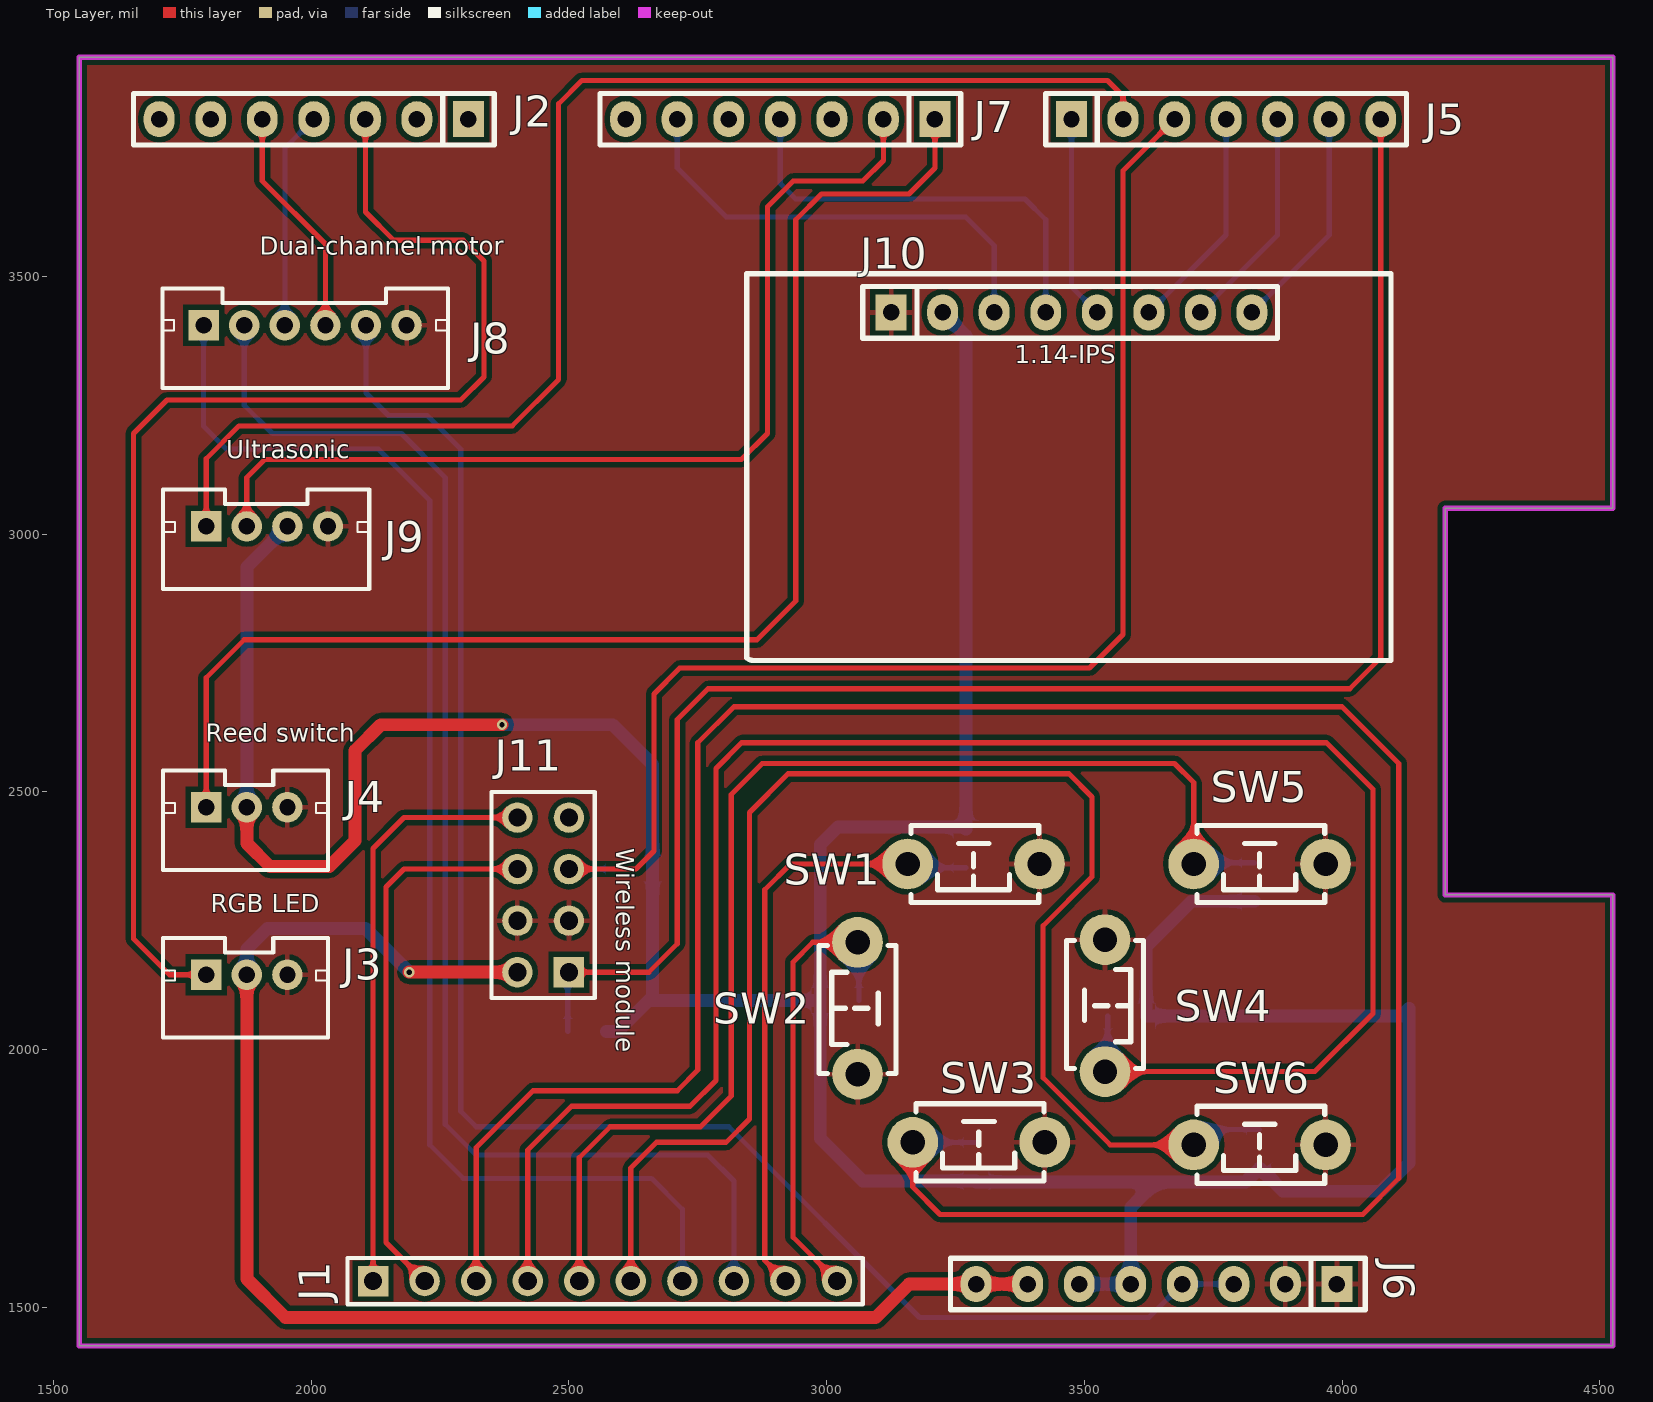
[diagram p0: Top Layer view]
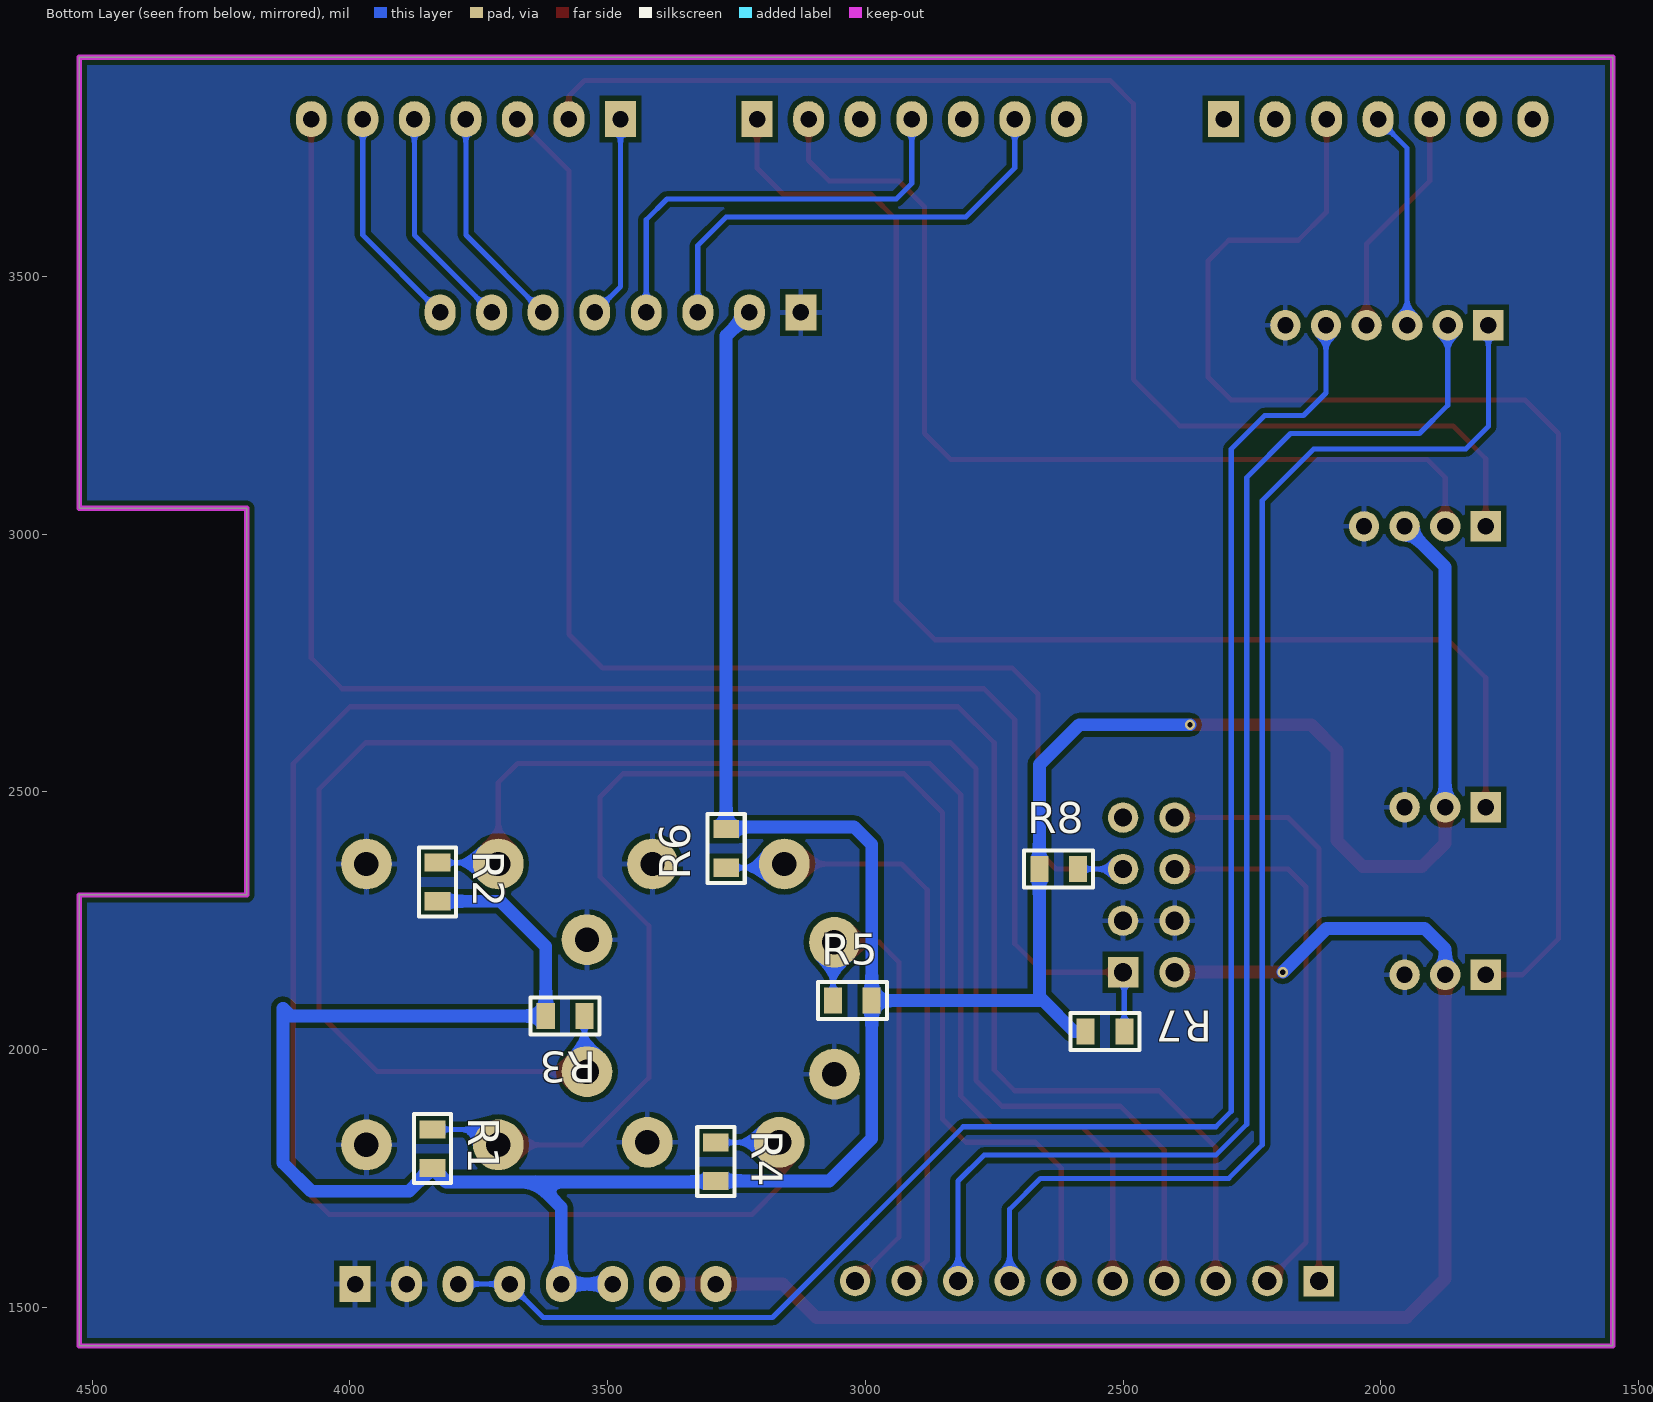
[diagram p1: Bottom Layer view, seen from below]
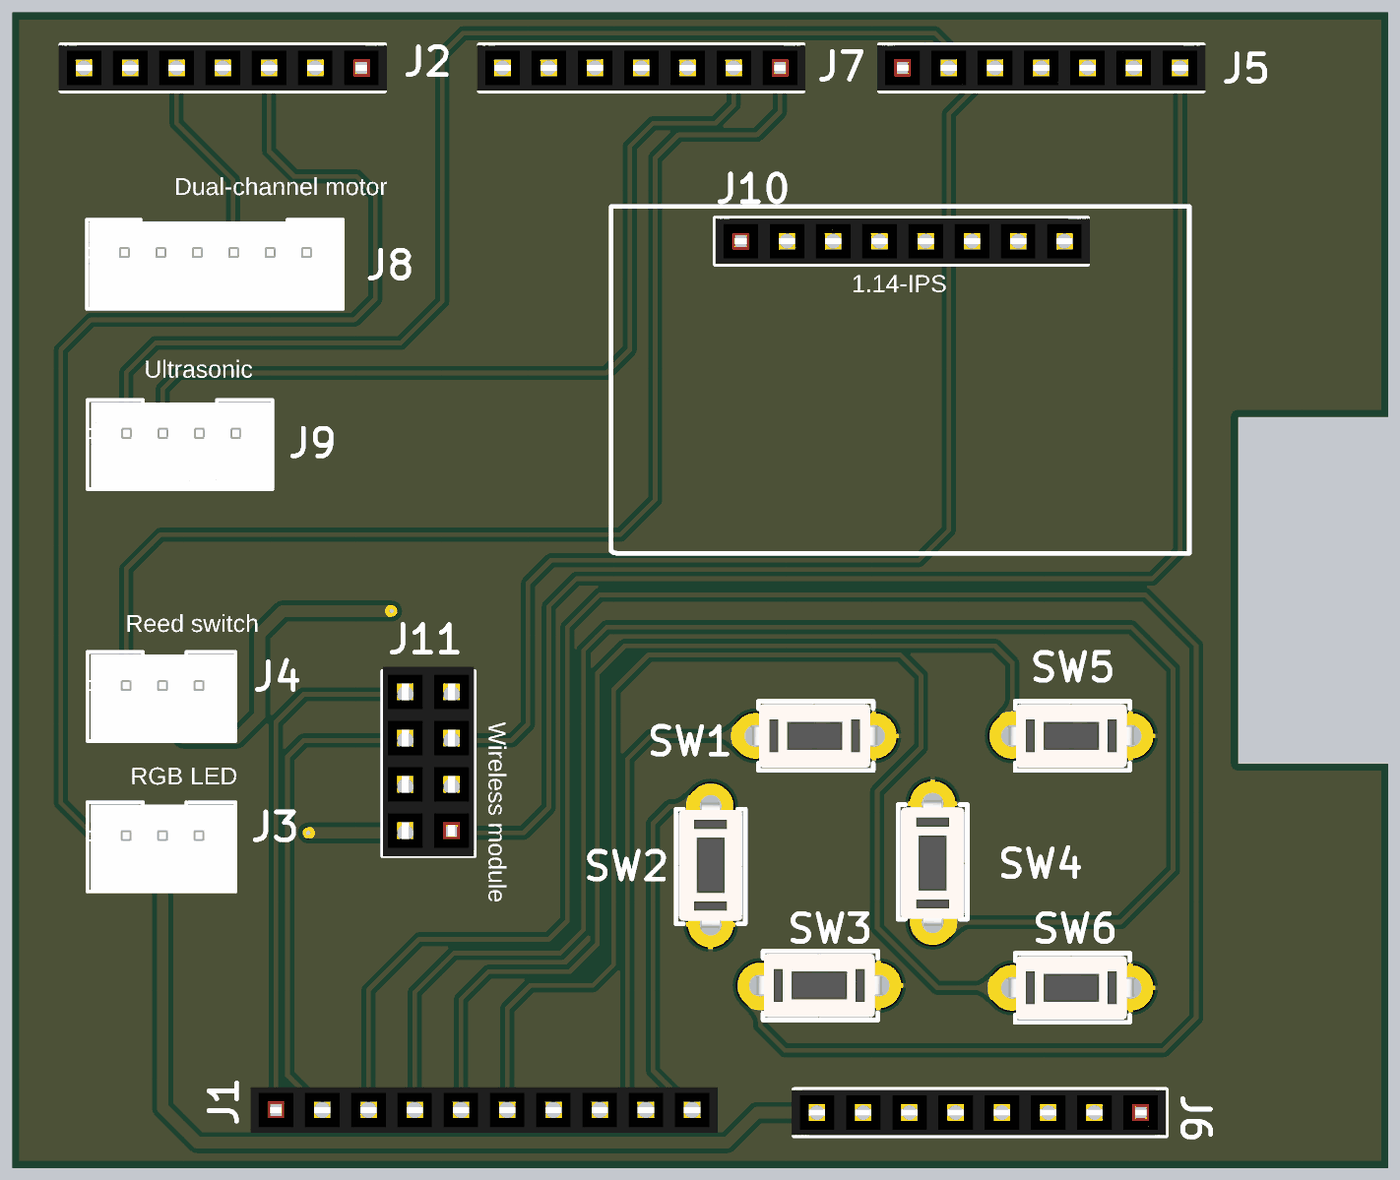
[diagram p2: 3D render of the assembled board from above, using the file's embedded part models]
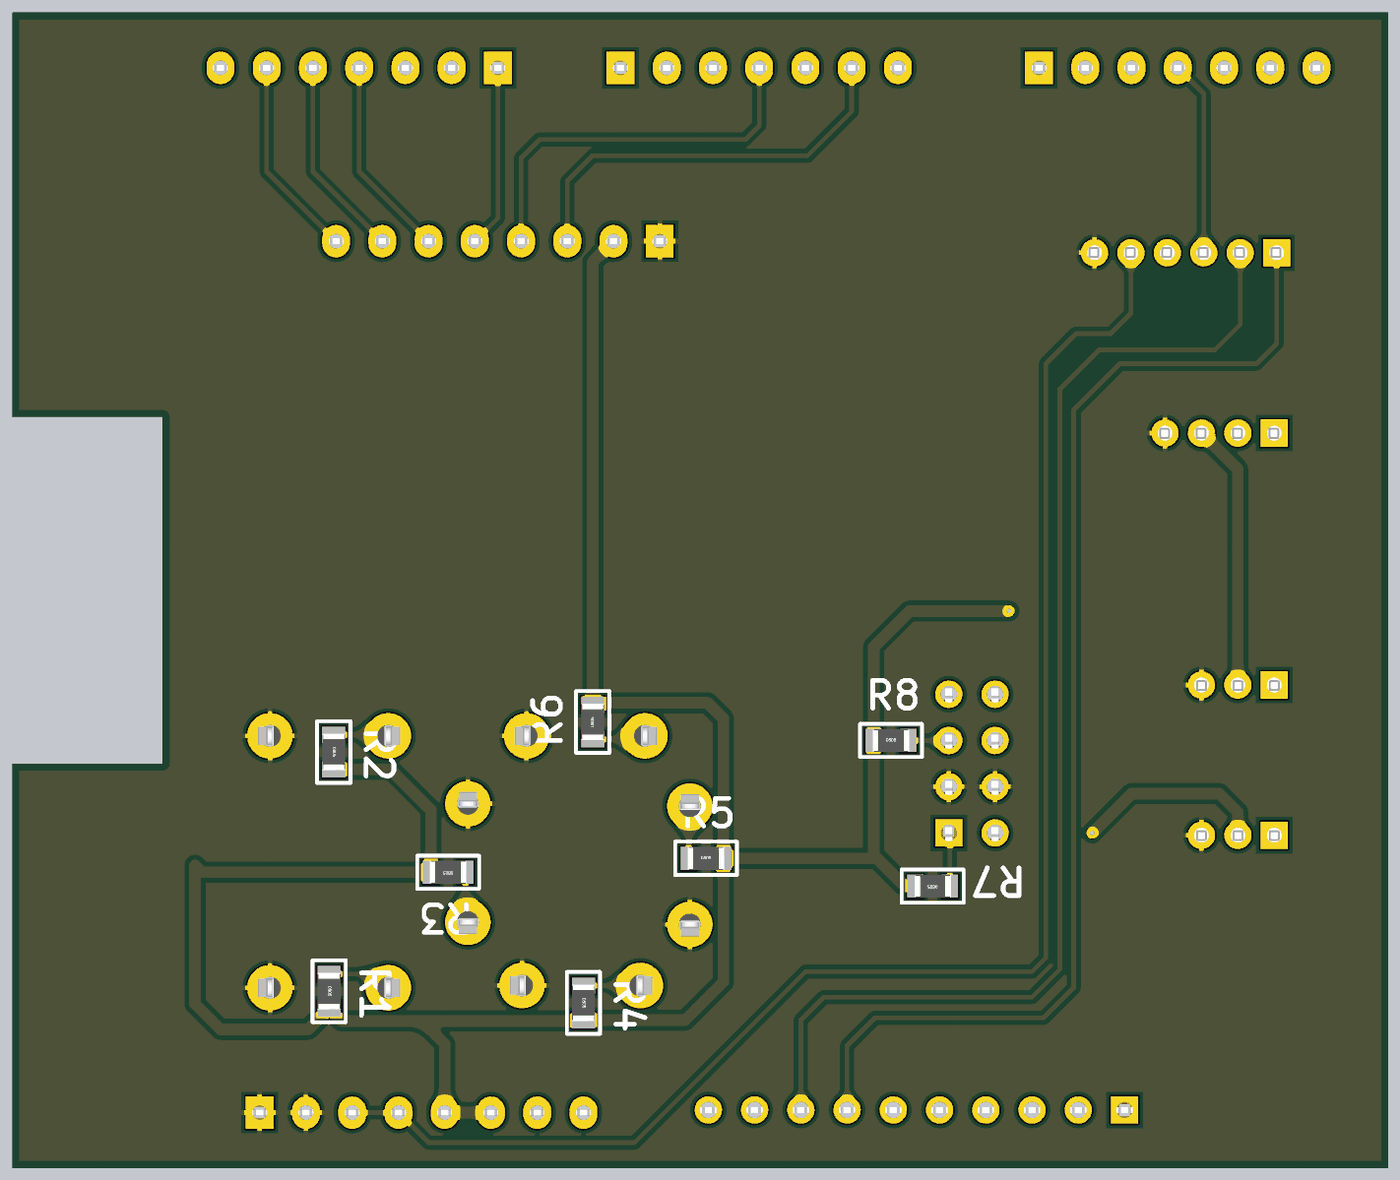
[diagram p3: 3D render of the assembled board from below, using the file's embedded part models]
# Altium PCB MISC80620.PcbDoc
Units mil, origin at the board's own origin, x right, y up, seen from the top; angles counter-clockwise.
Board outline 2975 x 2500 mil, 2 copper layers (Top Layer, Bottom Layer); 25 components, 35 nets, 99 pads, 2 vias.

## Layer stack, top to bottom (the 12.6 mil dielectric is the usual default, probably not edited)
Top Solder: solder mask 0.4, Solder Resist, Dk 3.5
Top Layer: signal copper 1.4
Dielectric 1: dielectric 12.6, FR-4, Dk 4.8
Bottom Layer: signal copper 1.4
Bottom Solder: solder mask 0.4, Solder Resist, Dk 3.5

## Board outline
1550,1425 1550,3925 4525,3925 4525,3050 4200,3050 4200,2300 4525,2300 4525,1425

## Design rules (kind name [scope] priority, off if disabled: settings)
Clearance [All] p1: gap=10
MinimumSolderMaskSliver [All] p1: minsoldermaskwidth=0
PolygonConnect [All] p1: connectstyle=Relief reliefconductorwidth=10 reliefentries=4 polygonreliefangle="90 Angle" airgapwidth=10
RoutingVias [All] p1: holewidth=28 width=50 viastyle="Through Hole" minholewidth=28 minwidth=50 maxholewidth=28 maxwidth=50
SilkToSilkClearance [All] p1: silktosilkclearance=0
SilkToSolderMaskClearance [IsPad] p1: minsilkscreentomaskgap=0 clearancetoexposedcopper=TRUE
SolderMaskExpansion [All] p1: expansion=4
Width [All] p1: maxlimit=30 minlimit=10 preferedwidth=10
27 further rules are at their usual default settings.

## Components (designator, comment, footprint, x,y, rotation, side; value= is the part's Value field where it differs from the comment)
J1 "Female HDR1X10" Fe-HDR1X10/2.54-S 2120,1550.78 r90 top
J2 "Female HDR1X7" Fe-HDR1X7/2.54-S 2305,3805 r270 top
J3 "PH2.0-3P" PH2.0-3P 1796.26,2145 r0 top
J4 "PH2.0-3P" PH2.0-3P 1796.26,2470 r0 top
J5 "Female HDR1X7" Fe-HDR1X7/2.54-S 3475,3805 r90 top
J6 "Female HDR1X8" Fe-HDR1X8/2.54-S 3990,1545 r270 top
J7 "Female HDR1X7" Fe-HDR1X7/2.54-S 3210,3805 r270 top
J8 "PH2.0-6P" PH2.0-6P 1791.26,3405 r0 top
J9 "PH2.0-4P" PH2.0-4P 1796.26,3015 r0 top
J10 "CON8" Fe-HDR1X8/2.54-S 3125,3430 r90 top
J11 "Female HDR2X4" Fe-HDR2X4/2.54-S 2500,2150 r90 top
R1 "4.7K" "R 0805_L" 3840,1807.6 r270 bottom
R2 "4.7K" "R 0805_L" 3830,2325 r270 bottom
R3 "4.7K" "R 0805_L" 3582.6,2065 r0 bottom
R4 "4.7K" "R 0805_L" 3290,1782.4 r270 bottom
R5 "4.7K" "R 0805_L" 3025,2095 r180 bottom
R6 "4.7K" "R 0805_L" 3270,2390 r90 bottom
R7 "10K" "R 0805_L" 2535,2035 r0 bottom
R8 "10K" "R 0805_L" 2625,2350 r180 bottom
SW1 "3x6x5" "TSW DIP-3*6*4.3" 3285,2360 r180 top
SW2 "3x6x5" "TSW DIP-3*6*4.3" 3060,2080 r90 top
SW3 "3x6x5" "TSW DIP-3*6*4.3" 3295,1820 r180 top
SW4 "3x6x5" "TSW DIP-3*6*4.3" 3540,2085 r270 top
SW5 "3x6x5" "TSW DIP-3*6*4.3" 3840,2360 r180 top
SW6 "3x6x5" "TSW DIP-3*6*4.3" 3840,1815 r180 top

## Footprints (in the part's own frame and the unit in brackets; to place one, negate y for a bottom-side part, rotate by r counter-clockwise, add the part's x,y. Pads: shape width x height; smd on the part's side, far side on the other; paste and mask are expansions set on the pad)
Fe-HDR1X7/2.54-S [mil]
  rect 70x60 hole 32: 1(0,0)
  oval 70x60 hole 32: 2(0,-100) 3(0,-200) 4(0,-300) 5(0,-400) 6(0,-500) 7(0,-600)
  silkscreen extent -50,-650 50,50, body extent -49,-655 49,55, height 126
Fe-HDR1X8/2.54-S [mil]
  rect 70x60 hole 32: 1(0,0)
  oval 70x60 hole 32: 2(0,-100) 3(0,-200) 4(0,-300) 5(0,-400) 6(0,-500) 7(0,-600) 8(0,-700)
  silkscreen extent -50,-750 50,55, body extent -49,-755 49,55, height 126
Fe-HDR1X10/2.54-S [mm]
  rect 1.5x1.5 hole 0.9: 1(0,0)
  round 1.5 hole 0.9: 2(0,-2.54) 3(0,-5.08) 4(0,-7.62) 5(0,-10.16) 6(0,-12.7) 7(0,-15.24) 8(0,-17.78) 9(0,-20.32) 10(0,-22.86)
  silkscreen extent -1.14,-24.13 1.14,1.27, body extent -1.25,-24.26 1.25,1.4, height 3.2
Fe-HDR2X4/2.54-S [mm] "Connector; Header; 4x2 Position"
  rect 1.5x1.5 hole 0.9: 1(0,0)
  round 1.5 hole 0.9: 2(0,2.54) 3(2.54,0) 4(2.54,2.54) 5(5.08,0) 6(5.08,2.54) 7(7.62,0) 8(7.62,2.54)
  silkscreen extent -1.27,-1.27 8.89,3.81, body extent -1.27,-1.23 9.14,3.77, height 8.5
PH2.0-3P [mm]
  rect 1.5x1.5 hole 0.8: 1(0,0)
  round 1.5 hole 0.8: 2(2,0) 3(4,0)
  silkscreen extent -2.13,-3.08 6,1.82, body extent -1.95,-3.02 5.95,1.68, height 6.01
PH2.0-4P [mm]
  rect 1.5x1.5 hole 0.8: 1(0,0)
  round 1.5 hole 0.8: 2(2,0) 3(4,0) 4(6,0)
  silkscreen extent -2.13,-3.08 8.03,1.82, body extent -1.93,-3.01 7.97,1.69, height 6.01
PH2.0-6P [mm]
  rect 1.5x1.5 hole 0.8: 1(0,0)
  round 1.5 hole 0.8: 2(2,0) 3(4,0) 4(6,0) 5(8,0) 6(10,0)
  silkscreen extent -2.03,-3.08 12.03,1.82, body extent -1.91,-2.98 11.99,1.71, height 6.01
"R 0805_L" [mil] "1/8W贴片电阻"
  rect 35x50 smd: 1(-37.4,0) 2(37.4,0)
  silkscreen extent -67,-36 67,36, body extent -39,-25 39,25, height 20
"TSW DIP-3*6*4.3" [mm] "3*6*4.3mm"
  round 2.5 hole 1.2: 1(3.25,0) 2(-3.25,0)
  silkscreen extent -3.21,-1.9 3.09,1.9, body extent -3.91,-1.75 3.91,1.75, height 4.31

## Part data
J10: library part "Female HDR1X8"
R1 R2 R3 R4 R5 R6 R7 R8: library part R, "SMD resistor"
SW1 SW2 SW3 SW4 SW5 SW6: library part "TSW 3x6", "3x6 tact switch"

## Via types
v1: diameter 20, hole 10, Top Layer to Bottom Layer, 2 vias

## Nets (pads, with @x,y where several pads share a name; then routed paths per layer and width w, separated by ;. In a path a pad name is that pad's centre, name@x,y a point inside that pad or via, vN(x,y) a via of type N, cw(c..) or ccw(c..) an arc to the next point about the centre after c; other vN are vias at no path point)
3V3: J4.2 J6.5 J6.6 J9.3 J10.2 R1.2 R2.2 R3.2 R4.2 R5.2 R6.2 R7.2 R8.1 | length 7240
  Top Layer w25: J4.2 1875,2400 1920,2355 2035,2355 2085,2405 2085,2580 2135,2630 v1(2370,2630)
  Bottom Layer w25: J4.2 1875,2936.26 J9.3 ; v1(2370,2630) 2585,2630 2662.4,2552.6 R8.1 2662.4,2102.4 2655,2095 ; R7.2 2595,2035 2655,2095 ; J10.2 3270,3385 R6.2 3265.68,2431.71 3021.71,2431.71 2987.6,2397.6 R5.2 ; J6.6 J6.5 3590,1693.29 3640,1743.29 ; R2.2 3707.6,2287.6 3620,2200 R3.2 4115,2065 4130,2080 4130,1780 4075,1725 3885.2,1725 R1.2 3813.09,1743.29 3640,1743.29 ; 2655,2095 R5.2 ; R5.2 2987.6,1827.4 3070,1745 R4.2 3290,1743.29 3640,1743.29
5V: J3.2 J6.7 J6.8 J11.2 | length 2789.8
  Top Layer w25: J3.2 1875,1555 1950,1480 3095,1480 3160,1545 J6.8 J6.7 ; v1(2190,2150) J11.2
  Bottom Layer w25: J3.2 1875,2195 1915,2235 2105,2235 v1(2190,2150)
A0: J1.7 J8.1 | length 2625.5
  Bottom Layer w10: J8.1 1791.26,3208.74 1835,3165 2130,3165 2230,3065 2230,1815 2295,1750 2660,1750 2720,1690 J1.7
A1: J1.8 J8.2 | length 2657.8
  Bottom Layer w10: J8.2 1870,3250 1925,3195 2175,3195 2260,3110 2260,1855 2320,1795 2770,1795 2820,1745 J1.8
A4: J1.9 R6.1 SW1.1 | length 1189.6
  Top Layer w10: J1.9 2880,1590.78 2880,2310 2930,2360 SW1.1
  Bottom Layer w10: SW1.1 3164.45,2352.6 R6.1
A5: J1.10 R5.1 SW2.1 | length 909.1
  Top Layer w10: J1.10 2935,1635.78 2935,2170 2972.95,2207.95 SW2.1
  Bottom Layer w10: SW2.1 3062.4,2205.55 R5.1
A7: J2.3 J3.1 | length 2550.2
  Top Layer w10: J3.1 1725,2145 1655,2215 1655,3195 1720,3260 2290,3260 2335,3305 2335,3530 2295,3570 2160,3570 2105,3625 J2.3
A11: J5.7 J11.1 R7.1 | length 3243.5
  Top Layer w10: J11.1 2655,2150 2710,2205 2710,2640 2770,2700 4015,2700 4075,2760 J5.7
  Bottom Layer w10: R7.1 2497.6,2147.6 J11.1
B0: J2.4 J8.3 | length 423.3
  Bottom Layer w10: J8.3 1948.74,3748.74 J2.4
B1: J2.5 J8.4 | length 450.7
  Top Layer w10: J2.5 1905,3685 2027.48,3562.52 J8.4
B3: J5.3 J11.5 R8.2 | length 2571.2
  Top Layer w10: J11.5 2630,2350 2665,2385 2665,2690 2715,2740 3510,2740 3575,2805 3575,3705 J5.3
  Bottom Layer w10: J11.5 R8.2
B4: J5.2 J9.1 | length 2584.7
  Top Layer w10: J9.1 1796.26,3146.26 1860,3210 2390,3210 2480,3300 2480,3835 2525,3880 3545,3880 3575,3850 J5.2
B7: J5.1 J10.5 | length 395.7
  Bottom Layer w10: J5.1 3475,3480 J10.5
B12: J7.7
B13: J7.6 J10.3 | length 902.1
  Bottom Layer w10: J7.6 2710,3710 2805,3615 3270,3615 3325,3560 J10.3
B14: J7.5
B15: J7.4 J10.4 | length 849
  Bottom Layer w10: J7.4 2910,3680 2940,3650 3385,3650 3425,3610 J10.4
C0: J1.1 J11.8 | length 1144.1
  Top Layer w10: J1.1 2120,2390 2180,2450 J11.8
C1: J1.2 J11.6 | length 1064.8
  Top Layer w10: J1.2 2145,1625.78 2145,2315 2180,2350 J11.6
C2: J1.3 R4.1 SW3.1 | length 4829.9
  Top Layer w10: J1.3 2320,1810 2430,1920 2710,1920 2750,1960 2750,2595 2820,2665 4000,2665 4110,2555 4110,1750 4040,1680 3220,1680 3167.05,1732.95 SW3.1
  Bottom Layer w10: SW3.1 3167.24,1819.8 R4.1
C3: J1.4 R3.1 SW4.1 | length 3725
  Top Layer w10: J1.4 2420,1805 2505,1890 2735,1890 2785,1940 2785,2545 2835,2595 3970,2595 4060,2505 4060,2070 3947.05,1957.05 SW4.1
  Bottom Layer w10: SW4.1 3545.2,1962.24 R3.1
C4: J1.5 R2.1 SW5.1 | length 2383.1
  Top Layer w10: J1.5 2520,1790 2580,1850 2755,1850 2815,1910 2815,2495 2875,2555 3675,2555 3712.05,2517.95 SW5.1
  Bottom Layer w10: SW5.1 3714.45,2362.4 R2.1
C5: J1.6 R1.1 SW6.1 | length 2868.9
  Top Layer w10: J1.6 2620,1770 2670,1820 2805,1820 2850,1865 2850,2460 2925,2535 3470,2535 3515,2490 3515,2335 3420,2240 3420,1945 3550,1815 SW6.1
  Bottom Layer w10: SW6.1 3742.05,1845 R1.1
D0: J5.6 J10.8 | length 437.1
  Bottom Layer w10: J10.8 3975,3580 J5.6
D4: J5.5 J10.7 | length 437.1
  Bottom Layer w10: J10.7 3875,3580 J5.5
D7: J5.4 J10.6 | length 437.1
  Bottom Layer w10: J10.6 3775,3580 J5.4
D8: J7.3
D9: J7.2 J9.2 | length 1922.5
  Top Layer w10: J9.2 1875,3110 1910,3145 2835,3145 2885,3195 2885,3635 2935,3685 3070,3685 3110,3725 J7.2
D10: J4.1 J7.1 | length 2603
  Top Layer w10: J4.1 1796.26,2721.26 1870,2795 2865,2795 2940,2870 2940,3610 2990,3660 3160,3660 3210,3710 J7.1
D11: J2.6
D12: J2.7
D13: J2.1
D14: J2.2
GND: J3.3 J4.3 J6.1 J6.2 J8.6 J9.4 J10.1 J11.3 J11.4 SW1.2 SW2.2 SW3.2 SW4.2 SW5.2 SW6.2
VIN: J6.3 J6.4 J8.5 | length 3337.7
  Bottom Layer w10: J8.5 2106.22,3273.78 2150,3230 2225,3230 2290,3165 2290,1880 2320,1850 2810,1850 3180,1480 3625,1480 J6.4 J6.3
pads on no net: J11.7

## Polygon pours and split planes (outlines as drawn)
GND on Bottom Layer "D" (solid, remove dead copper, pour order 0): 1310,4025 1325,4040 4960,4040 4960,1540 4535,1115 4395,1255 1075,1255
GND on Top Layer "D" (solid, remove dead copper, pour order 2): 1285,4030 4525,4030 4565,4070 4625,4010 4625,1285 1345,1285 1315,1315

## Keep-outs
Keep-Out Layer:
  lines w10: 1550,1425 4525,1425 4525,2300 4225,2300 4200,2300 4200,3050 4525,3050 4525,3925 1700,3925 1550,3925 1550,1425

## Silkscreen, mask and mechanical layers (free items; w line width, h text height)
Top Overlay:
  lines w10: 2970,2755 4095,2755 4095,3505 3045,3505 2845,3505 2845,2760 ccw(c2857.07,2772.07) 2857.07,2755 2980,2755
  text "Dual-channel motor" at 1900,3530 h60
  text "1.14-IPS" at 3365,3320 h60
  text "Ultrasonic" at 1835,3135 h60
  text "Reed switch" at 1795,2585 h60
  text "Wireless module" at 2580,2390 h60 r270
  text "RGB LED" at 1805,2255 h60